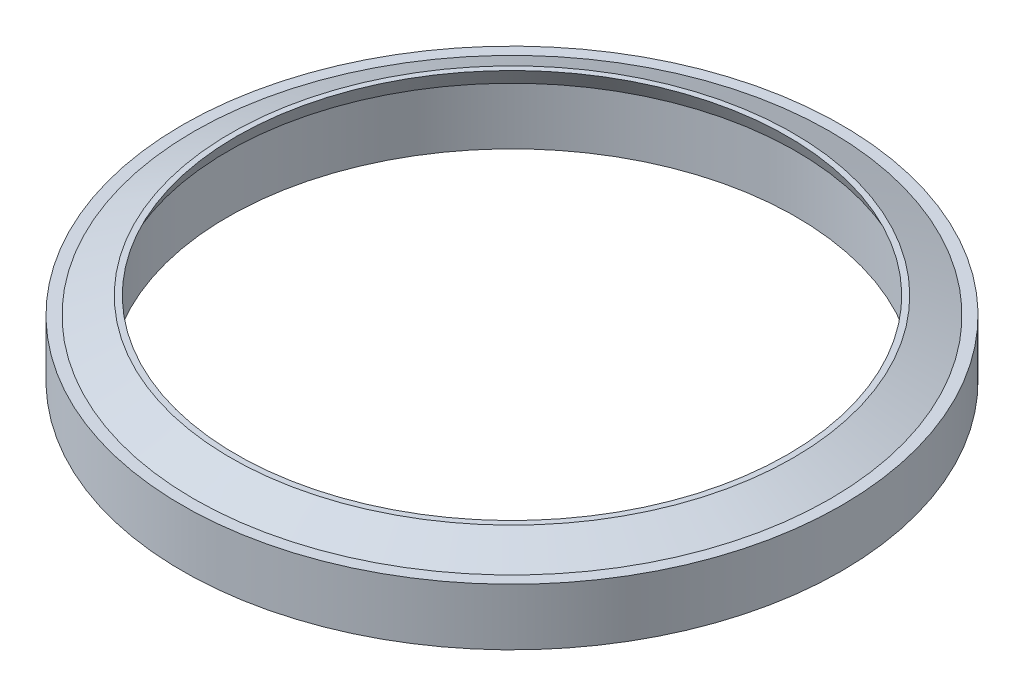
from build123d import *


with BuildPart() as part:
    # Sketch2 → Revolve1 (revolve)
    with BuildSketch(Plane.XY):
        Polygon((25, 0), (29, 0), (29, 5), (28, 5), (24.75, 6.5), (24.25, 6.5), (25, 5), align=None)
    revolve(axis=Axis((0, -1000, 0), (0, 1, 0)))


solid = part.part
